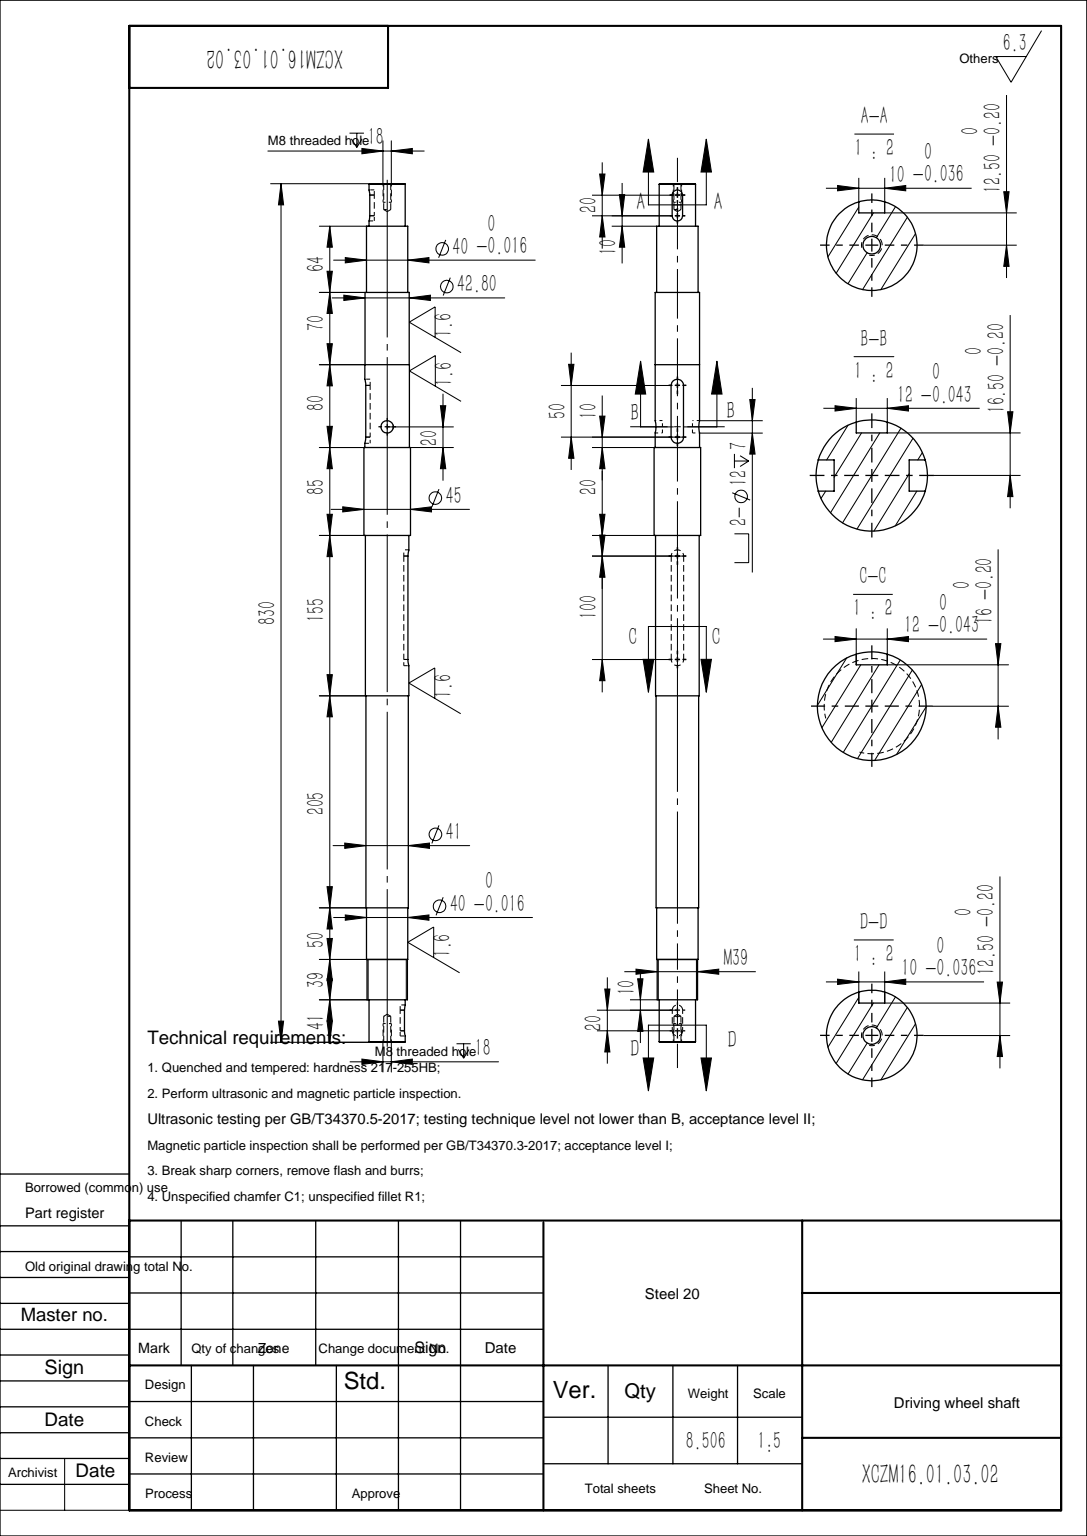
from build123d import *

# Parameters (mm, degrees)
M8_TAPPED_HOLE1_D       = 6.8
M8_TAPPED_HOLE1_DEPTH   = 25
M8_TAPPED_HOLE1_TIP     = 2.042926105
M8_TAPPED_HOLE2_D       = 6.8
M8_TAPPED_HOLE2_DEPTH   = 25
M8_TAPPED_HOLE2_TIP     = 2.042926105
CUT_EXTRUDE1_REACH      = 833.042
CUT_EXTRUDE1_END_RADIUS = 17.5
CUT_EXTRUDE2_REACH      = 833.197
CUT_EXTRUDE2_END_RADIUS = 21
CUT_EXTRUDE3_REACH      = 833.22
CUT_EXTRUDE3_END_RADIUS = 21.5
CUT_EXTRUDE4_REACH      = 833.042
CUT_EXTRUDE4_END_RADIUS = 17.5
CUT_EXTRUDE5_START      = -21.5
SKETCH11_R              = 6
CUT_EXTRUDE5_DEPTH      = 7
CHAMFER1_SIZE           = 0.5


with BuildPart() as part:
    # Sketch1 → Revolve1 (revolve)
    with BuildSketch(Plane.XY, mode=Mode.PRIVATE) as revolve1_sk:
        Polygon((0, 0), (0, 17.5), (41, 17.5), (41, 19.5), (80, 19.5), (80, 20), (130, 20), (130, 20.5), (335, 20.5), (335, 21), (490, 21), (490, 22.5), (575, 22.5), (575, 21.5), (655, 21.5), (655, 21.4), (725, 21.4), (725, 20), (789, 20), (789, 17.5), (830, 17.5), (830, 0), align=None)
    revolve(revolve1_sk.sketch.rotate(Axis((0, 0, 0), (-1, 0, 0)), 90), axis=Axis((0, 0, 0), (-1, 0, 0)))

    # M8 Tapped Hole1
    with Locations(Plane.ZY):
        with Locations((0, 0)):
            Hole(M8_TAPPED_HOLE1_D / 2, depth=M8_TAPPED_HOLE1_DEPTH)
            with Locations((0, 0, -(M8_TAPPED_HOLE1_DEPTH + M8_TAPPED_HOLE1_TIP / 2))):  # 118° drill point
                Cone(0, M8_TAPPED_HOLE1_D / 2, M8_TAPPED_HOLE1_TIP, mode=Mode.SUBTRACT)

    # M8 Tapped Hole2
    with Locations(Plane(origin=(830, 0, 0), x_dir=(0, 0, -1), z_dir=(1, 0, 0))):
        with Locations((0, 0)):
            Hole(M8_TAPPED_HOLE2_D / 2, depth=M8_TAPPED_HOLE2_DEPTH)
            with Locations((0, 0, -(M8_TAPPED_HOLE2_DEPTH + M8_TAPPED_HOLE2_TIP / 2))):  # 118° drill point
                Cone(0, M8_TAPPED_HOLE2_D / 2, M8_TAPPED_HOLE2_TIP, mode=Mode.SUBTRACT)

    # Cut-Extrude1: up to this cylinder (the profile starts inside it)
    cut_extrude1_end = Plane(origin=(21, 0, 0), z_dir=(1, 0, 0)) * Cylinder(CUT_EXTRUDE1_END_RADIUS, 1702.084, mode=Mode.PRIVATE)
    # Sketch6 → Cut-Extrude1 (cut, up to the surface)
    with BuildSketch(Plane.XY.offset(-12.5), mode=Mode.PRIVATE) as cut_extrude1_sk1:
        with BuildLine():
            Line((11, 5), (31, 5))
            ThreePointArc((31, 5), (36, 0), (31, -5))
            Line((31, -5), (11, -5))
            ThreePointArc((11, -5), (6, 0), (11, 5))
        make_face()
    cut_extrude1_tool1 = extrude(cut_extrude1_sk1.sketch, amount=-CUT_EXTRUDE1_REACH, mode=Mode.PRIVATE) & cut_extrude1_end
    add(cut_extrude1_tool1.solids().sort_by_distance((21, 0, -12.5))[0], mode=Mode.SUBTRACT)

    # Cut-Extrude2: up to this cylinder (the profile starts inside it)
    cut_extrude2_end = Plane(origin=(420, 0, 0), z_dir=(1, 0, 0)) * Cylinder(CUT_EXTRUDE2_END_RADIUS, 1709.394, mode=Mode.PRIVATE)
    # Sketch7 → Cut-Extrude2 (cut, up to the surface)
    with BuildSketch(Plane.XY.offset(-16), mode=Mode.PRIVATE) as cut_extrude2_sk1:
        with BuildLine():
            Line((370, 6), (470, 6))
            ThreePointArc((470, 6), (476, 0), (470, -6))
            Line((470, -6), (370, -6))
            ThreePointArc((370, -6), (364, 0), (370, 6))
        make_face()
    cut_extrude2_tool1 = extrude(cut_extrude2_sk1.sketch, amount=-CUT_EXTRUDE2_REACH, mode=Mode.PRIVATE) & cut_extrude2_end
    add(cut_extrude2_tool1.solids().sort_by_distance((420, 0, -16))[0], mode=Mode.SUBTRACT)

    # Cut-Extrude3: up to this cylinder (the profile starts inside it)
    cut_extrude3_end = Plane(origin=(610, 0, 0), z_dir=(1, 0, 0)) * Cylinder(CUT_EXTRUDE3_END_RADIUS, 1710.44, mode=Mode.PRIVATE)
    # Sketch9 → Cut-Extrude3 (cut, up to the surface)
    with BuildSketch(Plane.XY.offset(16.5), mode=Mode.PRIVATE) as cut_extrude3_sk1:
        with BuildLine():
            Line((585, 6), (635, 6))
            ThreePointArc((635, 6), (641, 0), (635, -6))
            Line((635, -6), (585, -6))
            ThreePointArc((585, -6), (579, 0), (585, 6))
        make_face()
    cut_extrude3_tool1 = extrude(cut_extrude3_sk1.sketch, amount=CUT_EXTRUDE3_REACH, mode=Mode.PRIVATE) & cut_extrude3_end
    add(cut_extrude3_tool1.solids().sort_by_distance((610, 0, 16.5))[0], mode=Mode.SUBTRACT)

    # Cut-Extrude4: up to this cylinder (the profile starts inside it)
    cut_extrude4_end = Plane(origin=(809, 0, 0), z_dir=(1, 0, 0)) * Cylinder(CUT_EXTRUDE4_END_RADIUS, 1702.084, mode=Mode.PRIVATE)
    # Sketch10 → Cut-Extrude4 (cut, up to the surface)
    with BuildSketch(Plane.XY.offset(12.5), mode=Mode.PRIVATE) as cut_extrude4_sk1:
        with BuildLine():
            Line((799, 5), (819, 5))
            ThreePointArc((819, 5), (824, 0), (819, -5))
            Line((819, -5), (799, -5))
            ThreePointArc((799, -5), (794, 0), (799, 5))
        make_face()
    cut_extrude4_tool1 = extrude(cut_extrude4_sk1.sketch, amount=CUT_EXTRUDE4_REACH, mode=Mode.PRIVATE) & cut_extrude4_end
    add(cut_extrude4_tool1.solids().sort_by_distance((809, 0, 12.5))[0], mode=Mode.SUBTRACT)

    # Sketch11 → Cut-Extrude5 (cut)
    with BuildSketch(Plane(origin=(0, 0, 0), x_dir=(1, 0, 0), z_dir=(0, 1, 0)).offset(CUT_EXTRUDE5_START)):
        with Locations(Location((595, 0, 0), (0, 0, 90))):
            Circle(SKETCH11_R)
    cut_extrude5 = extrude(amount=CUT_EXTRUDE5_DEPTH, mode=Mode.SUBTRACT)

    # Mirror1: Cut-Extrude5 across plane
    add(cut_extrude5.mirror(Plane.ZX), mode=Mode.SUBTRACT)

    # Chamfer1
    chamfer1_edges = [part.edges().sort_by_distance(p)[0] for p in [
        (830, 0, 17.5),
        (0, 0, 17.5),
    ]]
    chamfer(chamfer1_edges, length=CHAMFER1_SIZE)


solid = part.part
